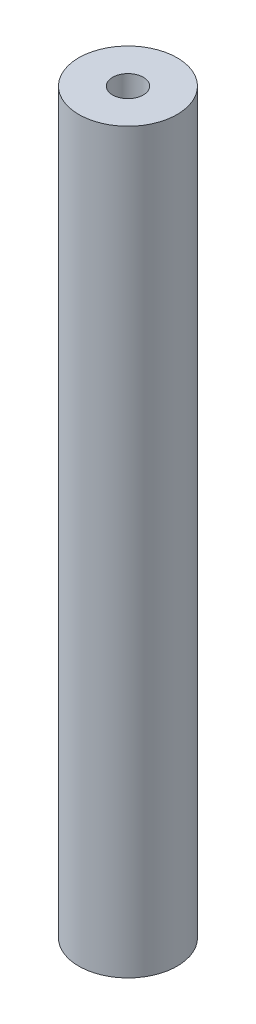
from build123d import *

# Parameters (mm, degrees)
SKETCH_1_W             = 8
SKETCH_1_H             = 120
HOLE_WIZARD_M6_1_D     = 5
HOLE_WIZARD_M6_1_DEPTH = 12
HOLE_WIZARD_M6_1_TIP   = 1.502151548
HOLE_WIZARD_M6_2_D     = 5
HOLE_WIZARD_M6_2_DEPTH = 12
HOLE_WIZARD_M6_2_TIP   = 1.502151548


with BuildPart() as part:
    # 草图1 → 旋转-薄壁1 (revolve)
    with BuildSketch(Plane.XY, mode=Mode.PRIVATE) as revolve_1_sk:
        with Locations((4, 0)):
            Rectangle(SKETCH_1_W, SKETCH_1_H)
    revolve(revolve_1_sk.sketch.rotate(Axis((0, 60, 0), (0, -1, 0)), 180), axis=Axis((0, 60, 0), (0, -1, 0)))

    # M6 螺纹孔的螺纹孔钻头1
    with Locations(Plane(origin=(0, 60, 0), x_dir=(1, 0, 0), z_dir=(0, 1, 0))):
        with Locations((0, 0)):
            Hole(HOLE_WIZARD_M6_1_D / 2, depth=HOLE_WIZARD_M6_1_DEPTH)
            with Locations((0, 0, -(HOLE_WIZARD_M6_1_DEPTH + HOLE_WIZARD_M6_1_TIP / 2))):  # 118° drill point
                Cone(0, HOLE_WIZARD_M6_1_D / 2, HOLE_WIZARD_M6_1_TIP, mode=Mode.SUBTRACT)

    # M6 螺纹孔的螺纹孔钻头2
    with Locations(Plane(origin=(0, -60, 0), x_dir=(-1, 0, 0), z_dir=(0, -1, 0))):
        with Locations((0, 0)):
            Hole(HOLE_WIZARD_M6_2_D / 2, depth=HOLE_WIZARD_M6_2_DEPTH)
            with Locations((0, 0, -(HOLE_WIZARD_M6_2_DEPTH + HOLE_WIZARD_M6_2_TIP / 2))):  # 118° drill point
                Cone(0, HOLE_WIZARD_M6_2_D / 2, HOLE_WIZARD_M6_2_TIP, mode=Mode.SUBTRACT)


solid = part.part
